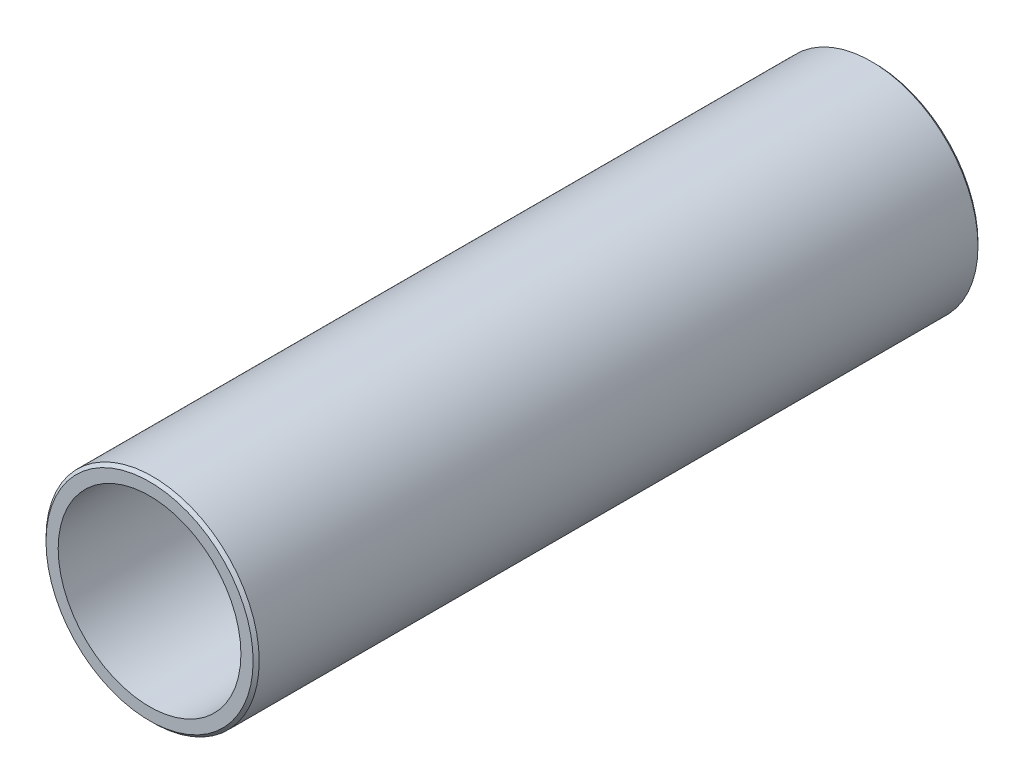
from build123d import *

# Parameters (mm, degrees)
SKETCH1_R           = 35
SKETCH1_R_2         = 30
BOSS_EXTRUDE1_DEPTH = 238
CHAMFER1_SIZE       = 1


with BuildPart() as part:
    # Sketch1 → Boss-Extrude1 (new body)
    with BuildSketch(Plane.XY):
        Circle(SKETCH1_R)
        Circle(SKETCH1_R_2, mode=Mode.SUBTRACT)
    extrude(amount=BOSS_EXTRUDE1_DEPTH)

    # Chamfer1
    chamfer1_edges = [part.edges().sort_by_distance(p)[0] for p in [
        (-35, 0, 0),
        (-35, 0, 238),
    ]]
    chamfer(chamfer1_edges, length=CHAMFER1_SIZE)


solid = part.part
